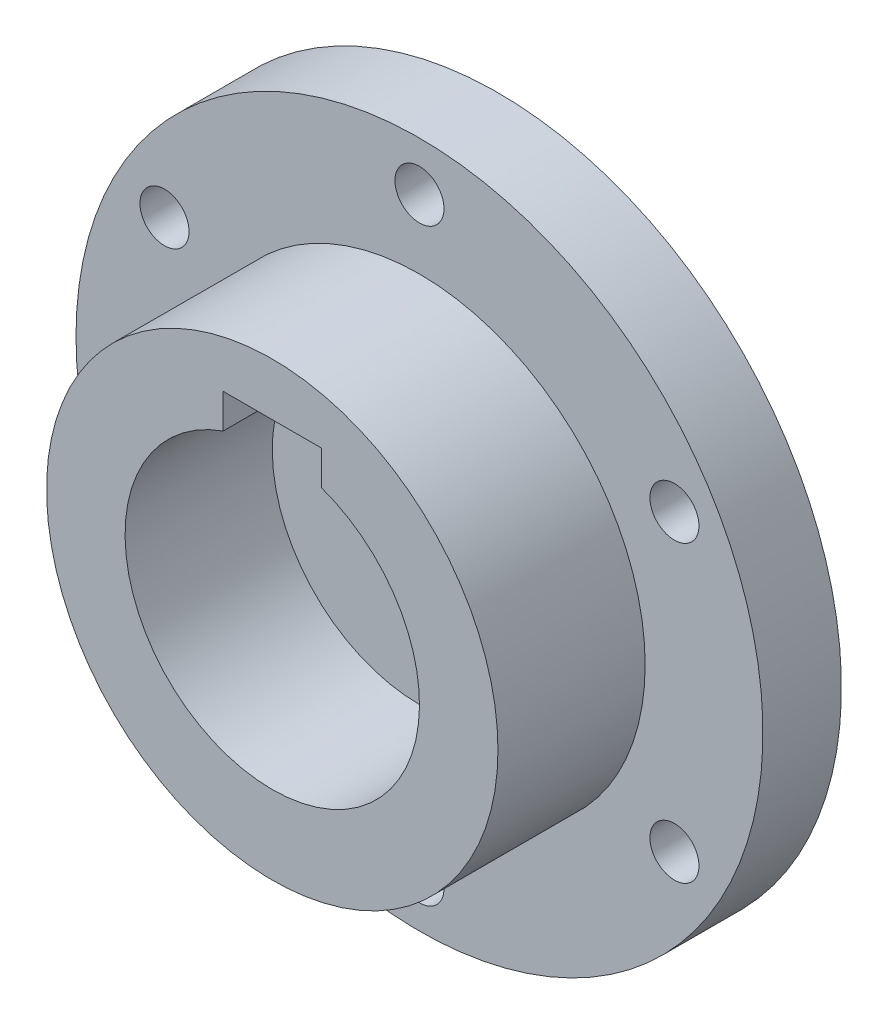
from build123d import *

# Parameters (mm, degrees)
SKETCH1_R               = 230
BOSS_EXTRUDE1_DEPTH     = 150
SKETCH2_R               = 350
BOSS_EXTRUDE2_DEPTH     = 80
CUT_EXTRUDE1_DEPTH      = 256
CUT_EXTRUDE1_DEPTH_BACK = 269
SKETCH3_R               = 25


with BuildPart() as part:
    # Sketch1 → Boss-Extrude1 (new body)
    with BuildSketch(Plane.XY):
        Circle(SKETCH1_R)
        with BuildLine():
            Line((-50, 141.421356237), (-50, 176.421356237))
            Line((-50, 176.421356237), (50, 176.421356237))
            Line((50, 176.421356237), (50, 141.421356237))
            ThreePointArc((50, 141.421356237), (0, -150), (-50, 141.421356237))
        make_face(mode=Mode.SUBTRACT)
    extrude(amount=-BOSS_EXTRUDE1_DEPTH)

    # Sketch2 → Boss-Extrude2 (add)
    with BuildSketch(Plane(origin=(0, 0, -150), x_dir=(-1, 0, 0), z_dir=(0, 0, -1))):
        Circle(SKETCH2_R)
    extrude(amount=BOSS_EXTRUDE2_DEPTH)

    # Sketch3 → Cut-Extrude1 (cut, two sides: drawn at the far end of the back side and taken through both)
    with BuildSketch(Plane(origin=(0, 0, -230), x_dir=(-1, 0, 0), z_dir=(0, 0, -1)).offset(-CUT_EXTRUDE1_DEPTH_BACK)):
        with Locations((0, 300)):
            Circle(SKETCH3_R)
        with Locations((259.807621135, 150)):
            Circle(SKETCH3_R)
        with Locations((259.807621135, -150)):
            Circle(SKETCH3_R)
        with Locations((0, -300)):
            Circle(SKETCH3_R)
        with Locations((-259.807621135, -150)):
            Circle(SKETCH3_R)
        with Locations((-259.807621135, 150)):
            Circle(SKETCH3_R)
    extrude(amount=CUT_EXTRUDE1_DEPTH + CUT_EXTRUDE1_DEPTH_BACK, mode=Mode.SUBTRACT)


solid = part.part
